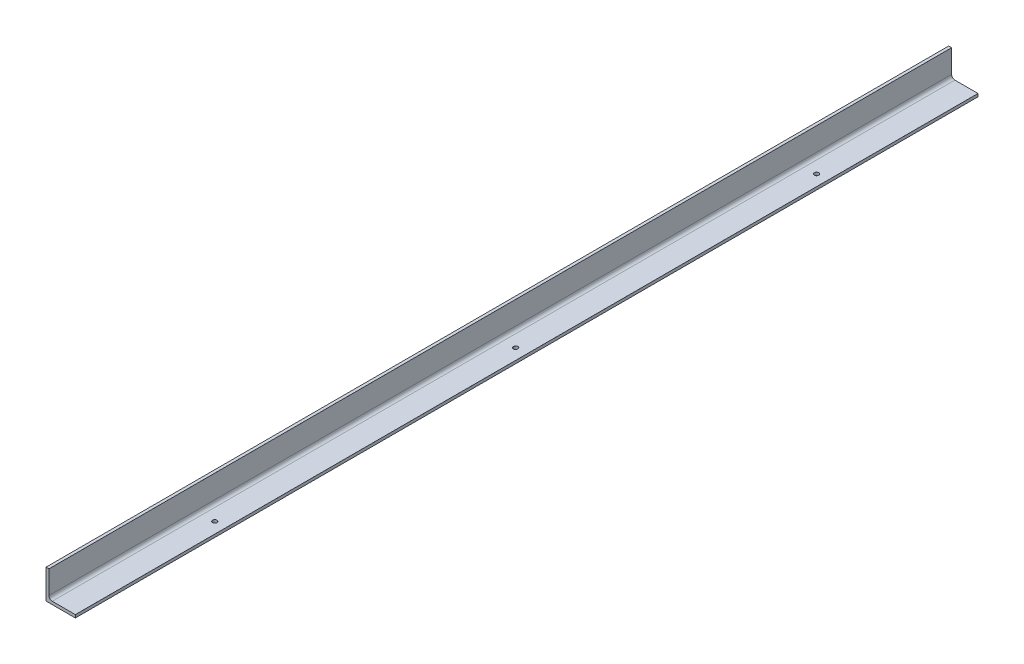
from build123d import *

# Parameters (mm, degrees)
EXTRUDE_1_DEPTH        = 1230
HOLE_WIZARD_6_0_6_1_D  = 6
PATTERN_LINEAR_1_COUNT = 3
PATTERN_LINEAR_1_PITCH = 410


with BuildPart() as part:
    # 草图1 → 拉伸1 (new body)
    with BuildSketch(Plane.XY):
        with BuildLine():
            Line((0, 0), (0, 40))
            Line((0, 40), (3.99, 40))
            ThreePointArc((3.99, 40), (3.997071068, 39.997071068), (4, 39.99))
            Line((4, 39.99), (4, 8.5))
            ThreePointArc((4, 8.5), (5.318019485, 5.318019485), (8.5, 4))
            Line((8.5, 4), (39.99, 4))
            ThreePointArc((39.99, 4), (39.997071068, 3.997071068), (40, 3.99))
            Line((40, 3.99), (40, 0))
            Line((40, 0), (0, 0))
        make_face()
    extrude(amount=EXTRUDE_1_DEPTH)

    # Ø6.0 (6) 直径孔1 (through all)
    with Locations(Plane(origin=(0, 0, 0), x_dir=(-1, 0, 0), z_dir=(0, -1, 0))):
        with Locations((-25, -205)):
            hole_wizard_6_0_6_1 = Hole(HOLE_WIZARD_6_0_6_1_D / 2)

    # 阵列(线性)1: Ø6.0 (6) 直径孔1 ×3
    with Locations(*[(0, 0, i * PATTERN_LINEAR_1_PITCH) for i in range(1, PATTERN_LINEAR_1_COUNT)]):
        add(hole_wizard_6_0_6_1, mode=Mode.SUBTRACT)


solid = part.part
